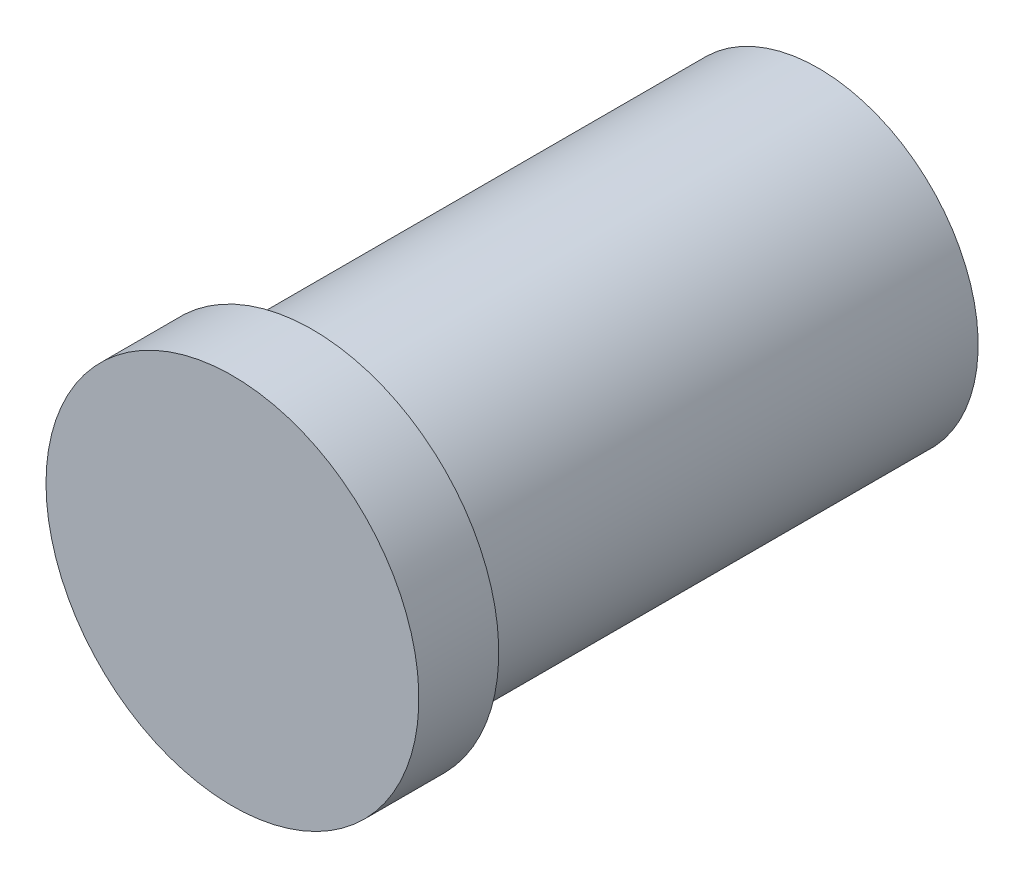
from build123d import *


with BuildPart() as part:
    # Sketch1 → Revolve1 (revolve)
    with BuildSketch(Plane(origin=(0, 0, 0), x_dir=(1, 0, 0), z_dir=(0, 1, 0)), mode=Mode.PRIVATE) as revolve1_sk:
        Polygon((0, 0), (7, 0), (7, 3), (6, 3), (6, 22), (0, 22), align=None)
    revolve(revolve1_sk.sketch.rotate(Axis((0, 0, -22), (0, 0, 1)), 180), axis=Axis((0, 0, -22), (0, 0, 1)))


solid = part.part
